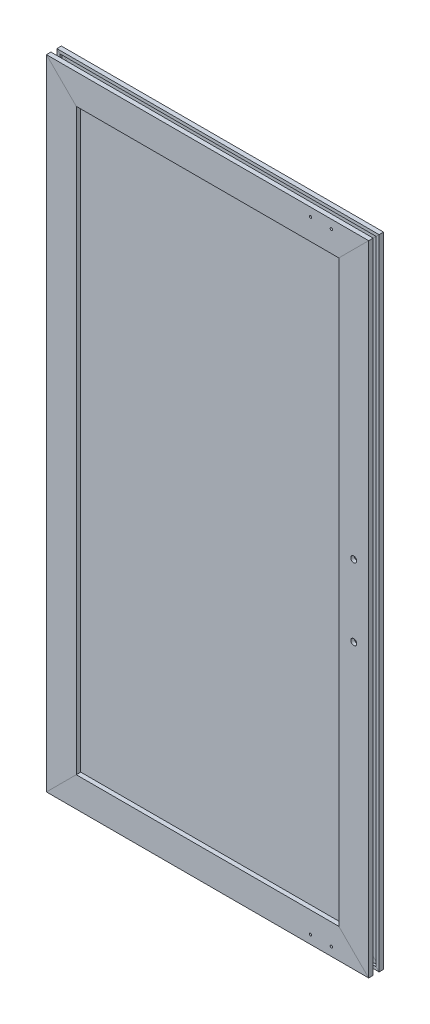
SolidWorks part; units mm, degrees
material "铝型材"
ref_plane "前视基准面" through (0, 0, 0) normal (0, 0, 1) x (1, 0, 0)
ref_plane "上视基准面" through (0, 0, 0) normal (0, 1, 0) x (1, 0, 0)
ref_plane "右视基准面" through (0, 0, 0) normal (1, 0, 0) x (0, 0, -1)
sketch "草图13" plane through (0, 0, 0) normal (0, 0, 1) x (1, 0, 0)
  line L1 (-196, -408) -> (196, -408)
  line L2 (-196, -408) -> (-196, 408)
  line L3 (-196, 408) -> (196, 408)
  line L4 (196, -408) -> (196, 408)
  line L5 (-196, -408) -> (196, 408) construction
  line L6 (-196, 408) -> (196, -408) construction
  point P0 (0, 0)
  dimension "D1" = 392
  dimension "D2" = 816
other "铝型材 2040A(1)"
ref_plane "基准面3" through (-196, 408, 0) normal (1, 0, 0) x (0, 1, 0)
sketch "草图19" plane through (-196, 408, 0) normal (1, 0, 0) x (0, 1, 0)
  line L0 (9, 4) -> (6, 4)
  line L1 (9, 4) -> (9, 7)
  line L2 (6, -4) -> (6, 4)
  line L3 (16, 7) -> (9, 7)
  line L4 (9, -4) -> (6, -4)
  line L5 (16, 4) -> (16, 7)
  line L6 (9, -7) -> (9, -4)
  line L7 (20, 4) -> (16, 4)
  line L8 (16, -7) -> (9, -7)
  line L9 (20, 10) -> (20, 4)
  line L10 (16, -7) -> (16, -4)
  line L11 (-20, 10) -> (20, 10)
  line L12 (20, -4) -> (16, -4)
  line L13 (-20, 4) -> (-20, 10)
  line L14 (20, -4) -> (20, -10)
  line L15 (-20, 4) -> (-16, 4)
  line L16 (20, -10) -> (-20, -10)
  line L17 (-16, 4) -> (-16, 7)
  line L18 (-20, -10) -> (-20, -4)
  line L19 (-16, 7) -> (-9, 7)
  line L20 (-20, -4) -> (-16, -4)
  line L21 (-9, 4) -> (-9, 7)
  line L22 (-16, -7) -> (-16, -4)
  line L23 (-9, 4) -> (-6, 4)
  line L24 (-16, -7) -> (-9, -7)
  line L25 (-6, -4) -> (-6, 4)
  line L26 (-9, -7) -> (-9, -4)
  line L27 (-9, -4) -> (-6, -4)
  circle A0 centre (0, 0) radius 3.25
  point P0 (0, 0)
sketch "草图14" plane through (0, 0, 0) normal (0, 0, 1) x (1, 0, 0)
  line L0 (202, 414) -> (205, 417) construction
  line L1 (-189.5, -401.5) -> (189.5, -401.5)
  line L2 (-189.5, -401.5) -> (-189.5, 401.5)
  line L3 (-189.5, 401.5) -> (189.5, 401.5)
  line L4 (189.5, -401.5) -> (189.5, 401.5)
  line L5 (-189.5, -401.5) -> (189.5, 401.5) construction
  line L6 (-189.5, 401.5) -> (189.5, -401.5) construction
  line L8 (176, 388) -> (-176, 388) construction
  point P0 (0, 0)
  dimension "D1" = 13.5
extrude "凸台-拉伸1" add sketch "草图14" along normal mid plane 4 separate body
hole_wizard "M4 螺纹孔2" positions "草图24" profile "草图25" tap size "M4" standard "GB"
sketch "草图24" plane through (0, 0, 10) normal (0, 0, -1) x (-1, 0, 0)
  line L0 (-166, 416.5) -> (-138, 416.5) construction
  line L7 (0, 0) -> (81.0682, 0) construction
  line L10 (-216, 428) -> (216, 428) construction
  line L11 (-216, -428) -> (-216, 428) construction
  point P0 (-166, 416.5)
  point P2 (-138, 416.5)
  point P29 (-138, -416.5)
  point P30 (-166, -416.5)
  dimension "D1" = 28
  dimension "D2" = 11.5
  dimension "D3" = 50
cosmetic thread "孔螺蚊线3"
cosmetic thread "孔螺蚊线4"
cosmetic thread "孔螺蚊线9"
cosmetic thread "孔螺蚊线10"
sketch "草图25" plane through (166, 416.5, 10) normal (1, 0, 0) x (0, -1, 0)
  line L0 (0, 0) -> (0, 11.0914)
  line L1 (0, 11.0914) -> (1.65, 10.1)
  line L2 (1.65, 10.1) -> (1.65, 0)
  line L5 (1.65, 0) -> (0, 0)
  line L10 (0, 11.0914) -> (-1.65, 10.1) construction
  line L11 (0, -6.35) -> (0, 107.95) construction
  dimension "螺纹孔钻头直径" = 3.3
  dimension "螺纹孔钻头深度" = 10.1
  dimension "导头角度" = 118
hole_wizard "打孔尺寸(%根据)开槽圆柱头螺钉的类型1" positions "草图26" profile "草图27" counterbore size "M4" standard "GB" end condition through all
sketch "草图26" plane through (0, 0, 10) normal (0, 0, 1) x (1, 0, 0)
  line L0 (0, 0) -> (50000, 0) construction
  line L1 (196, 424) -> (196, -49576) construction
  line L2 (216, 428) -> (176, 388) construction
  point P0 (196, 48)
  point P2 (196, -48)
  point P14 (196, 408)
  dimension "D1" = 96
sketch "草图27" plane through (196, 48, 10) normal (1, 0, 0) x (0, -1, 0)
  line L0 (0, 0) -> (0, 20)
  line L1 (0, 20) -> (2.25, 20)
  line L3 (2.25, 20) -> (2.25, 4.6)
  line L4 (2.25, 4.6) -> (4, 4.6)
  line L5 (4, 4.6) -> (4, 0)
  line L7 (4, 0) -> (0, 0)
  line L11 (0, -6.35) -> (0, 107.95) construction
  dimension "通孔孔直径" = 4.5
  dimension "通孔孔深度" = 20
  dimension "柱形沉头孔直径" = 8
  dimension "柱形沉头孔深度" = 4.6
hole_wizard "M6 螺纹孔1" positions "草图28" profile "草图29" tap size "M6" standard "GB"
sketch "草图28" plane through (0, 0, -10) normal (0, 0, -1) x (-1, 0, 0)
  line L0 (0, 0) -> (50000, 0) construction
  line L1 (196, 424) -> (196, -49576) construction
  line L2 (176, 388) -> (216, 428) construction
  line L3 (-216, 428) -> (216, 428) construction
  line L4 (196, -469.5) -> (196, 49530.5) construction
  point P0 (196, 368)
  point P2 (196, 331)
  point P12 (196, 408)
  point P19 (196, -368)
  point P20 (196, -331)
  dimension "D1" = 60
  dimension "D2" = 37
sketch "草图29" plane through (-196, 368, -10) normal (1, 0, 0) x (0, 1, 0)
  line L0 (0, 0) -> (0, 18.5022)
  line L1 (0, 18.5022) -> (2.5, 17)
  line L2 (2.5, 17) -> (2.5, 0)
  line L5 (2.5, 0) -> (0, 0)
  line L10 (0, 18.5022) -> (-2.5, 17) construction
  line L11 (0, -6.35) -> (0, 107.95) construction
  dimension "螺纹孔钻头直径" = 5
  dimension "螺纹孔钻头深度" = 17
  dimension "导头角度" = 118
cosmetic thread "孔螺蚊线5"
cosmetic thread "孔螺蚊线6"
cosmetic thread "孔螺蚊线7"
cosmetic thread "孔螺蚊线8"
